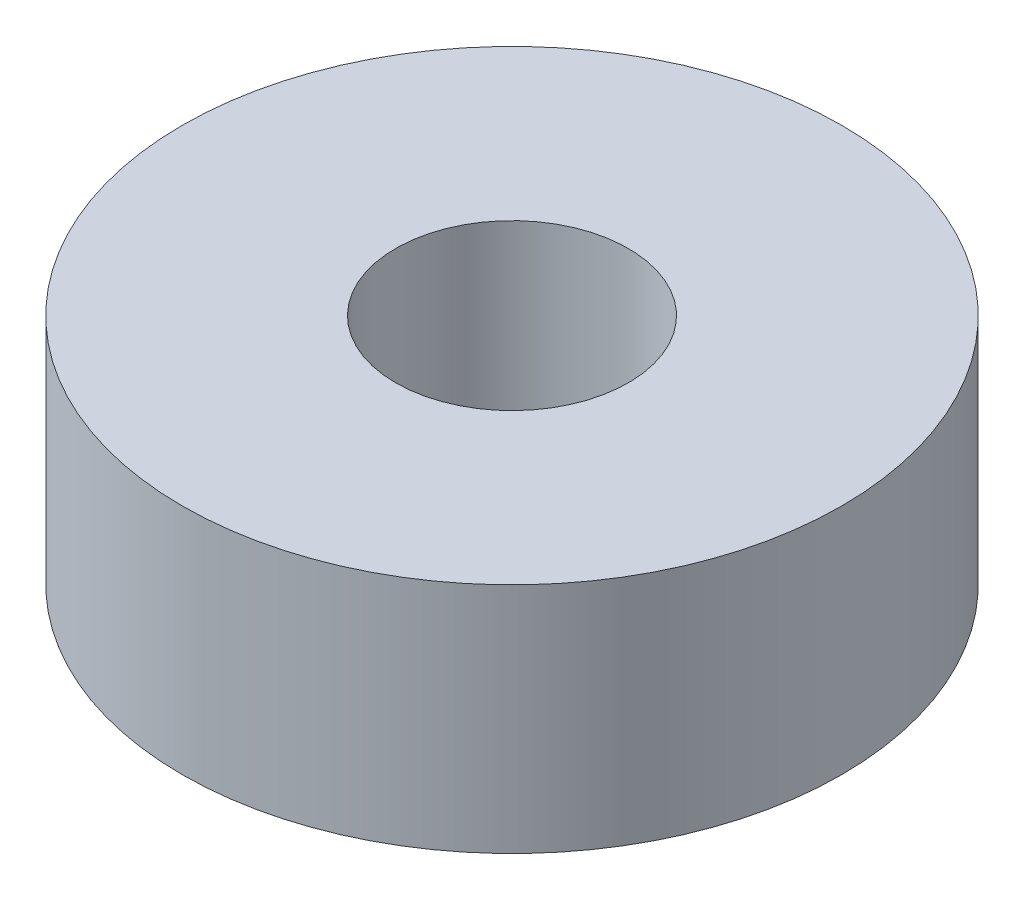
SolidWorks part; units mm, degrees
ref_plane "Front Plane" through (0, 0, 0) normal (0, 0, 1) x (1, 0, 0)
ref_plane "Top Plane" through (0, 0, 0) normal (0, 1, 0) x (1, 0, 0)
ref_plane "Right Plane" through (0, 0, 0) normal (1, 0, 0) x (0, 0, -1)
sketch "Sketch1" plane through (0, 0, 0) normal (0, 1, 0) x (1, 0, 0)
  circle A0 centre (0, 0) radius 3
  circle A1 centre (0, 0) radius 8.5
  dimension "D1" = 17
  dimension "D2" = 6
extrude "Boss-Extrude1" add sketch "Sketch1" along normal blind 6
